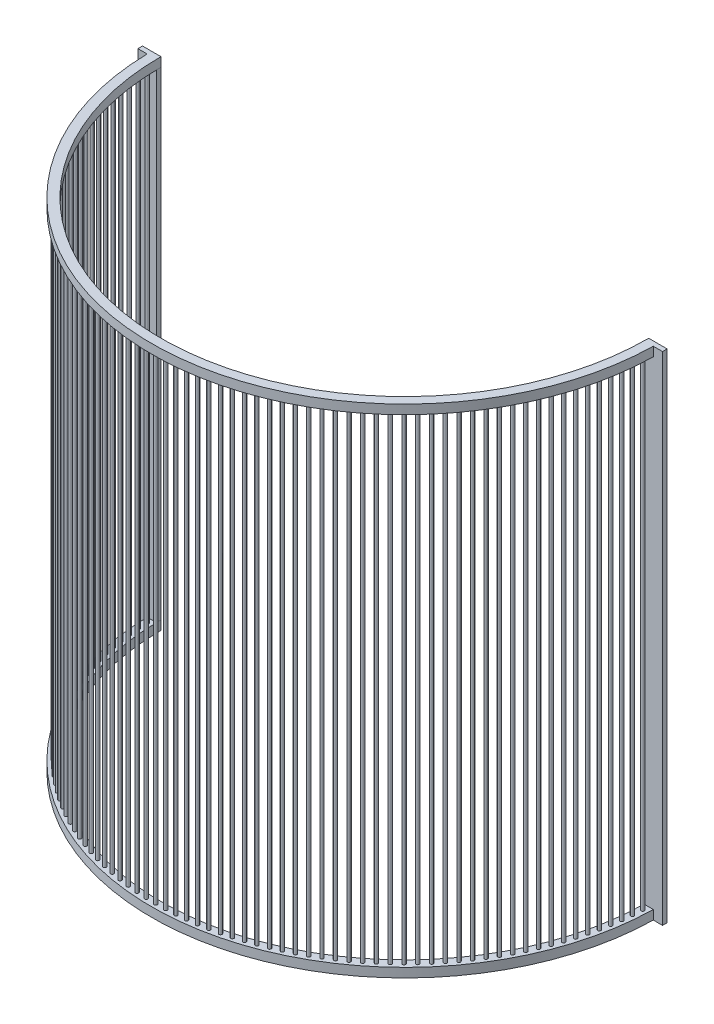
from build123d import *

# Parameters (mm, degrees)
BOSS_EXTRUDE1_DEPTH = 10
SKETCH2_W           = 20
SKETCH2_H           = 5
BOSS_EXTRUDE2_DEPTH = 260
SKETCH3_R           = 1.717629463
BOSS_EXTRUDE3_DEPTH = 520
CIRPATTERN1_COUNT   = 80
CIRPATTERN1_ANGLE   = 177.75


with BuildPart() as part:
    # Sketch1 → Boss-Extrude1 (new body)
    with BuildSketch(Plane(origin=(0, 0, 0), x_dir=(1, 0, 0), z_dir=(0, 1, 0))):
        with BuildLine():
            Line((265, 0), (275, 0))
            Line((275, 0), (285, 0))
            Line((285, 0), (285, -5))
            Line((285, -5), (274.954541697, -5))
            ThreePointArc((274.954541697, -5), (0, -275), (-274.954541697, -5))
            Line((-274.954541697, -5), (-285, -5))
            Line((-285, -5), (-285, 0))
            Line((-285, 0), (-275, 0))
            Line((-275, 0), (-265, 0))
            ThreePointArc((-265, 0), (0, -265), (265, 0))
        make_face()
    boss_extrude1 = extrude(amount=BOSS_EXTRUDE1_DEPTH)

    # Sketch2 → Boss-Extrude2 (add)
    with BuildSketch(Plane(origin=(0, 10, 0), x_dir=(1, 0, 0), z_dir=(0, 1, 0))):
        with Locations((-275, -2.5)):
            Rectangle(SKETCH2_W, SKETCH2_H)
        with Locations((275, -2.5)):
            Rectangle(SKETCH2_W, SKETCH2_H)
    boss_extrude2 = extrude(amount=BOSS_EXTRUDE2_DEPTH)

    # Mirror2: Boss-Extrude2 across plane
    add(boss_extrude2.mirror(Plane.ZX.offset(270)))

    # Mirror3: Boss-Extrude1 across plane
    add(boss_extrude1.mirror(Plane.ZX.offset(270)))

    # Sketch3 → Boss-Extrude3 (add)
    with BuildSketch(Plane(origin=(0, 10, 0), x_dir=(1, 0, 0), z_dir=(0, 1, 0))):
        with Locations(Location((-269.814751265, -10, 0), (0, 0, 90))):
            Circle(SKETCH3_R)
    boss_extrude3 = extrude(amount=BOSS_EXTRUDE3_DEPTH)

    # CirPattern1: Boss-Extrude3 ×80 about axis
    cirpattern1_axis = Axis((0, 0, 0), (0, 1, 0))
    for i in range(1, CIRPATTERN1_COUNT):
        add(boss_extrude3.rotate(cirpattern1_axis, i * CIRPATTERN1_ANGLE / (CIRPATTERN1_COUNT - 1)))


solid = part.part
